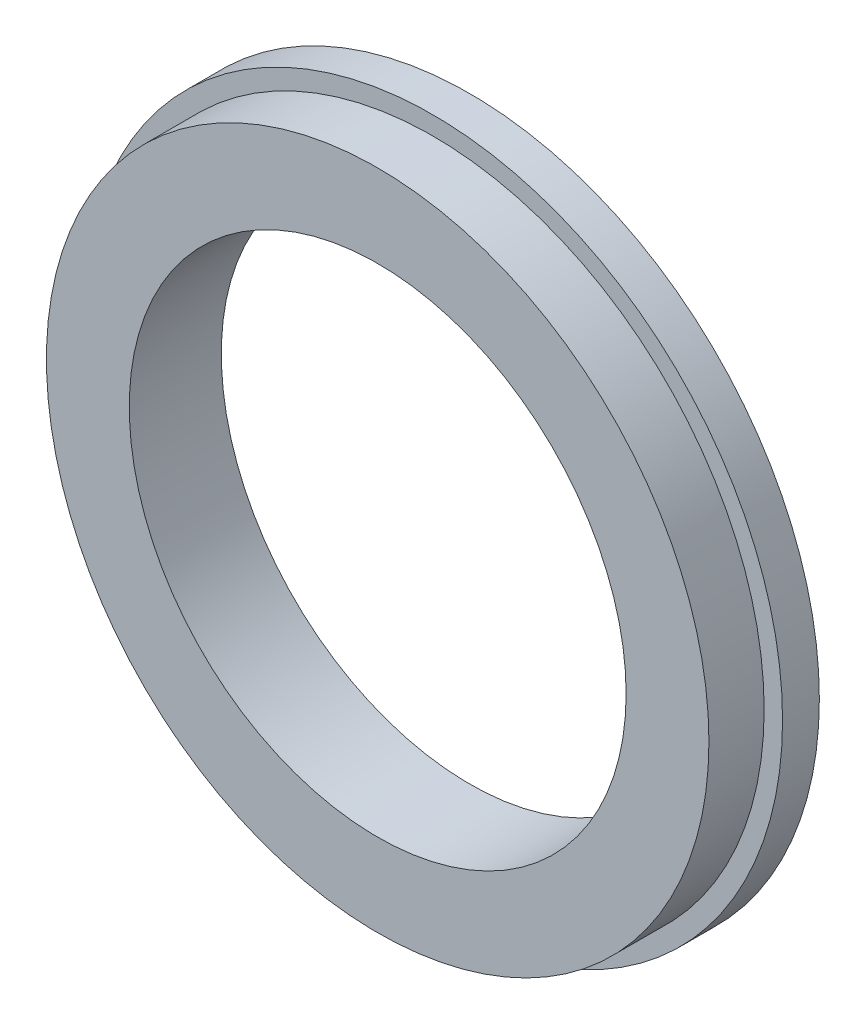
SolidWorks part; units mm, degrees
ref_plane "Front Plane" through (0, 0, 0) normal (0, 0, 1) x (1, 0, 0)
ref_plane "Top Plane" through (0, 0, 0) normal (0, 1, 0) x (1, 0, 0)
ref_plane "Right Plane" through (0, 0, 0) normal (1, 0, 0) x (0, 0, -1)
sketch "Sketch1" plane through (0, 0, 0) normal (0, 0, 1) x (1, 0, 0)
  circle A0 centre (0, 0) radius 95
  circle A1 centre (0, 0) radius 67.5
extrude "Boss-Extrude1" add sketch "Sketch1" along normal blind 10
sketch "Sketch2" plane through (0, 0, 10) normal (0, 0, 1) x (1, 0, 0)
  circle A0 centre (0, 0) radius 90
  circle A1 centre (0, 0) radius 67.5
extrude "Boss-Extrude2" add sketch "Sketch2" along normal blind 15
sketch "Sketch5" plane through (0, 0, 0) normal (0, 0, -1) x (-1, 0, 0)
  circle A0 centre (0, 0) radius 80.5 construction
  circle A1 centre (0, 80.5) radius 5.9
  circle A2 centre (69.715, 40.25) radius 5.9
  circle A3 centre (69.715, -40.25) radius 5.9
  circle A4 centre (0, -80.5) radius 5.9
  circle A5 centre (-69.715, -40.25) radius 5.9
  circle A6 centre (-69.715, 40.25) radius 5.9
  point P17 (0, 0)
  dimension "D1" = 6
hole_wizard "M12 Tapped Hole2" positions "3DSketch2" profile "Sketch6" tap size "M12" standard "Gb"
sketch3d "3DSketch2"
  point P0 (0, 80.5, 0)
  point P3 (69.715, 40.25, 0)
  point P6 (69.715, -40.25, 0)
  point P9 (0, -80.5, 0)
  point P12 (-69.715, -40.25, 0)
  point P15 (-69.715, 40.25, 0)
sketch "Sketch6" plane through (0, 80.5, 0) normal (1, 0, 0) x (0, 1, 0)
  line L0 (0, 0) -> (0, 13.0644)
  line L1 (0, 13.0644) -> (5.1, 10)
  line L2 (5.1, 10) -> (5.1, 0)
  line L5 (5.1, 0) -> (0, 0)
  line L10 (0, 13.0644) -> (-5.1, 10) construction
  line L11 (0, -6.35) -> (0, 107.95) construction
  dimension "螺纹孔钻头直径" = 10.2
  dimension "螺纹孔钻头深度" = 10
  dimension "导头角度" = 118
cosmetic thread "Cosmetic Thread7" parameters "D1"=10, "D2"=12
cosmetic thread "Cosmetic Thread8" parameters "D1"=10, "D2"=12
cosmetic thread "Cosmetic Thread9" parameters "D1"=10, "D2"=12
cosmetic thread "Cosmetic Thread10" parameters "D1"=10, "D2"=12
cosmetic thread "Cosmetic Thread11" parameters "D1"=10, "D2"=12
cosmetic thread "Cosmetic Thread12" parameters "D1"=10, "D2"=12
